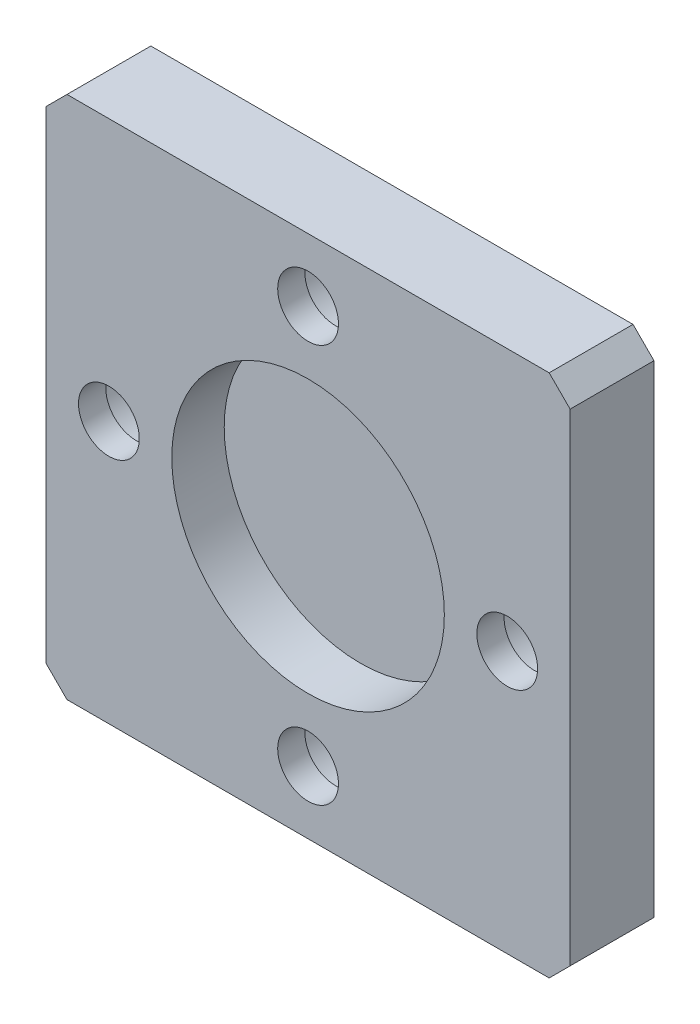
from build123d import *

# Parameters (mm, degrees)
SKETCH_1_W                   = 50
SKETCH_1_H                   = 50
EXTRUDE_1_DEPTH              = 4
SKETCH_2_R                   = 13
CUT_EXTRUDE_1_DEPTH          = 5
HOLE_WIZARD_M5_1_D           = 5.8
HOLE_WIZARD_M5_1_CBORE_D     = 10
HOLE_WIZARD_M5_1_CBORE_DEPTH = 5.4
CHAMFER_1_SIZE               = 2


with BuildPart() as part:
    # 草图1 → 凸台-拉伸1 (new, symmetric)
    with BuildSketch(Plane.XY):
        Rectangle(SKETCH_1_W, SKETCH_1_H)
    extrude(amount=EXTRUDE_1_DEPTH, both=True)

    # 草图2 → 切除-拉伸1 (cut)
    with BuildSketch(Plane.XY.offset(4)):
        Circle(SKETCH_2_R)
    extrude(amount=-CUT_EXTRUDE_1_DEPTH, mode=Mode.SUBTRACT)

    # M5 六角凹头螺钉的柱形沉头孔1 (through all)
    with Locations(Plane(origin=(0, 0, -4), x_dir=(1, 0, 0), z_dir=(0, 0, -1))):
        with Locations((-19, 0), (0, -19), (19, 0), (0, 19)):
            CounterBoreHole(HOLE_WIZARD_M5_1_D / 2, HOLE_WIZARD_M5_1_CBORE_D / 2, HOLE_WIZARD_M5_1_CBORE_DEPTH)

    # 倒角1
    chamfer_1_edges = [part.edges().sort_by_distance(p)[0] for p in [
        (25, -25, 0),
        (-25, -25, 0),
        (-25, 25, 0),
        (25, 25, 0),
    ]]
    chamfer(chamfer_1_edges, length=CHAMFER_1_SIZE)


solid = part.part
